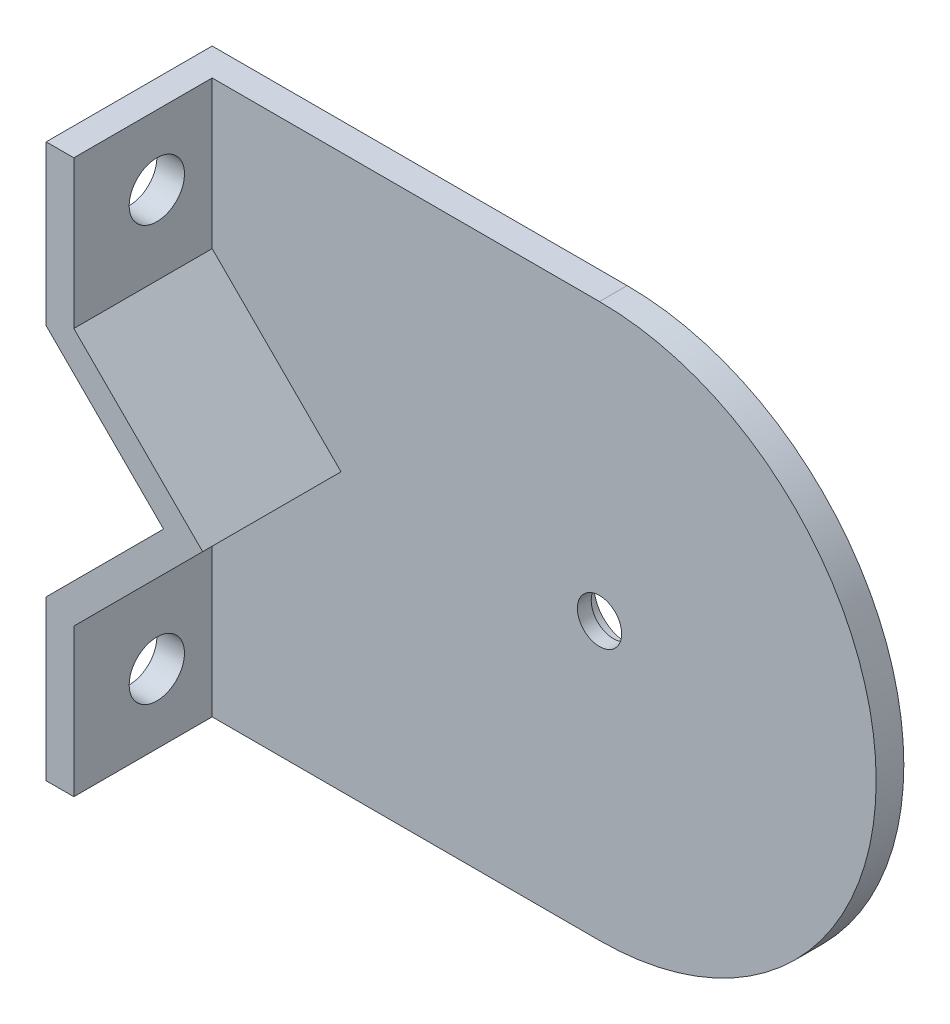
SolidWorks part; units mm, degrees
ref_plane "前视基准面" through (0, 0, 0) normal (0, 0, 1) x (1, 0, 0)
ref_plane "上视基准面" through (0, 0, 0) normal (0, 1, 0) x (1, 0, 0)
ref_plane "右视基准面" through (0, 0, 0) normal (1, 0, 0) x (0, 0, -1)
sketch "草图1" plane through (0, 0, 0) normal (0, 0, 1) x (1, 0, 0)
  line L0 (0, 100) -> (-150, 100)
  line L1 (-150, 100) -> (-150, -100)
  line L2 (-150, -100) -> (0, -100)
  arc A0 (0, -100) -> (0, 100) centre (0, 0) ccw
  circle A1 centre (0, 0) radius 8
  point P2 (-150, 0)
  dimension "D1" = 16
  dimension "D2" = 200
  dimension "D3" = 150
extrude "凸台-拉伸1" add sketch "草图1" along normal blind 10
sketch "草图2" plane through (0, 0, 10) normal (0, 0, 1) x (1, 0, 0)
  line L0 (-150, 42.4264) -> (-150, 100)
  line L1 (-150, 100) -> (-150, -100) construction
  line L2 (-150, 42.4264) -> (-107.5736, 0)
  line L3 (-107.5736, 0) -> (-150, -42.4264)
  line L4 (-150, 100) -> (-140, 100)
  line L5 (0, 100) -> (-150, 100) construction
  line L6 (-140, 100) -> (-140, 46.5685)
  line L7 (-140, 46.5685) -> (-93.4315, 0)
  line L8 (-93.4315, 0) -> (-140, -46.5685)
  line L9 (-140, -46.5685) -> (-140, -100)
  line L10 (-150, -100) -> (0, -100) construction
  line L11 (-140, -100) -> (-150, -100)
  line L12 (-150, -100) -> (-150, -42.4264)
  dimension "D1" = 60
  dimension "D2" = 90
  dimension "D3" = 0
  dimension "D4" = 60
  dimension "D5" = 10
  dimension "D6" = 10
  dimension "D7" = 10
  dimension "D8" = 10
extrude "凸台-拉伸2" add sketch "草图2" along normal blind 50
sketch "草图3" plane through (0, 0, 10) normal (0, 0, 1) x (1, 0, 0)
  line L3 (-150, -42.4264) -> (-107.5736, 0)
  line L4 (-107.5736, 0) -> (-150, 42.4264)
  line L5 (-150, 42.4264) -> (-150, -42.4264)
  line L6 (-150, -42.4264) -> (-107.5736, 0)
  line L7 (-107.5736, 0) -> (-150, 42.4264)
  line L8 (-150, 42.4264) -> (-150, -42.4264)
  dimension "D1" = 0
extrude "切除-拉伸1" cut sketch "草图3" against normal through all
sketch "草图4" plane through (-150, 0, 0) normal (-1, 0, 0) x (0, 0, 1)
  line L2 (60, 100) -> (0, 100) construction
  line L3 (60, -100) -> (0, -100) construction
  circle A0 centre (30, -75) radius 10
  circle A1 centre (30, 75) radius 10
  dimension "D1" = 25
  dimension "D2" = 25
extrude "切除-拉伸2" cut sketch "草图4" against normal blind 40
sketch "草图6" plane through (0, 0, 0) normal (0, 0, -1) x (-1, 0, 0)
  circle A0 centre (0, 0) radius 12
  dimension "D1" = 24
extrude "切除-拉伸4" cut sketch "草图6" against normal blind 5
